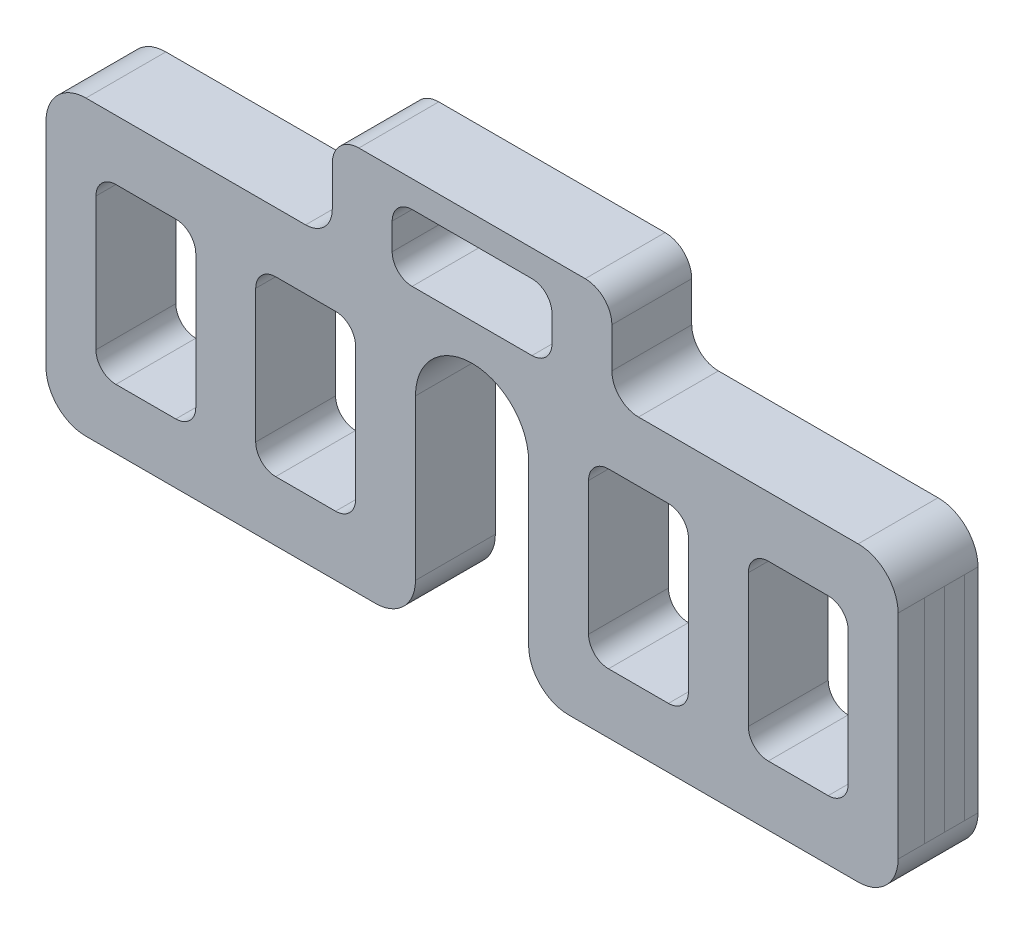
from build123d import *

# Parameters (mm, degrees)
BOSS_EXTRUDE1_DEPTH  = 30
SKETCH5_W            = 75
SKETCH5_H            = 130
CUT_EXTRUDE3_DEPTH   = 433.897216438
FILLET2_R            = 15
FILLET2_OF_MIRROR3_R = 15
FILLET3_R            = 30


with BuildPart() as part:
    # Sketch1 → Boss-Extrude1 (new, symmetric)
    with BuildSketch(Plane.XY):
        with BuildLine():
            Line((42.5, 0), (320, 0))
            Line((320, 0), (320, 220))
            Line((320, 220), (125, 220))
            ThreePointArc((125, 220), (110.857864376, 225.857864376), (105, 240))
            Line((105, 240), (105, 270))
            ThreePointArc((105, 270), (99.142135624, 284.142135624), (85, 290))
            Line((85, 290), (-85, 290))
            ThreePointArc((-85, 290), (-99.142135624, 284.142135624), (-105, 270))
            Line((-105, 270), (-105, 240))
            ThreePointArc((-105, 240), (-110.857864376, 225.857864376), (-125, 220))
            Line((-125, 220), (-320, 220))
            Line((-320, 220), (-320, 0))
            Line((-320, 0), (-42.5, 0))
            Line((-42.5, 0), (-42.5, 150))
            ThreePointArc((-42.5, 150), (0, 192.5), (42.5, 150))
            Line((42.5, 150), (42.5, 0))
        make_face()
        with BuildLine():
            Line((45, 220), (-45, 220))
            ThreePointArc((-45, 220), (-55.606601718, 224.393398282), (-60, 235))
            Line((-60, 235), (-60, 255))
            ThreePointArc((-60, 255), (-55.606601718, 265.606601718), (-45, 270))
            Line((-45, 270), (45, 270))
            ThreePointArc((45, 270), (55.606601718, 265.606601718), (60, 255))
            Line((60, 255), (60, 235))
            ThreePointArc((60, 235), (55.606601718, 224.393398282), (45, 220))
        make_face(mode=Mode.SUBTRACT)
    extrude(amount=BOSS_EXTRUDE1_DEPTH, both=True)

    # Sketch5 → Cut-Extrude3 (cut, symmetric)
    with BuildSketch(Plane.XY):
        with Locations((-245, 110)):
            Rectangle(SKETCH5_W, SKETCH5_H)
        with Locations((-125, 110)):
            Rectangle(SKETCH5_W, SKETCH5_H)
    cut_extrude3 = extrude(amount=CUT_EXTRUDE3_DEPTH, both=True, mode=Mode.SUBTRACT)

    # Fillet2
    fillet2_edges = [part.edges().sort_by_distance(p)[0] for p in [
        (-207.5, 175, 0),
        (-207.5, 45, 0),
        (-282.5, 45, 0),
        (-282.5, 175, 0),
        (-87.5, 175, 0),
        (-87.5, 45, 0),
        (-162.5, 45, 0),
        (-162.5, 175, 0),
    ]]
    fillet(fillet2_edges, radius=FILLET2_R)

    # Mirror3: Cut-Extrude3 across plane
    add(cut_extrude3.mirror(Plane(origin=(0, 0, 0), x_dir=(0, 0, 1), z_dir=(1, 0, 0))), mode=Mode.SUBTRACT)

    # Fillet2 of Mirror3
    fillet2_of_mirror3_edges = [part.edges().sort_by_distance(p)[0] for p in [
        (207.5, 175, 0),
        (207.5, 45, 0),
        (282.5, 45, 0),
        (282.5, 175, 0),
        (87.5, 175, 0),
        (87.5, 45, 0),
        (162.5, 45, 0),
        (162.5, 175, 0),
    ]]
    fillet(fillet2_of_mirror3_edges, radius=FILLET2_OF_MIRROR3_R)

    # Fillet3
    fillet3_edges = [part.edges().sort_by_distance(p)[0] for p in [
        (-42.5, 0, 0),
        (-320, 0, 0),
        (-320, 220, 0),
        (320, 220, 0),
        (320, 0, 0),
        (42.5, 0, 0),
    ]]
    fillet(fillet3_edges, radius=FILLET3_R)


solid = part.part
